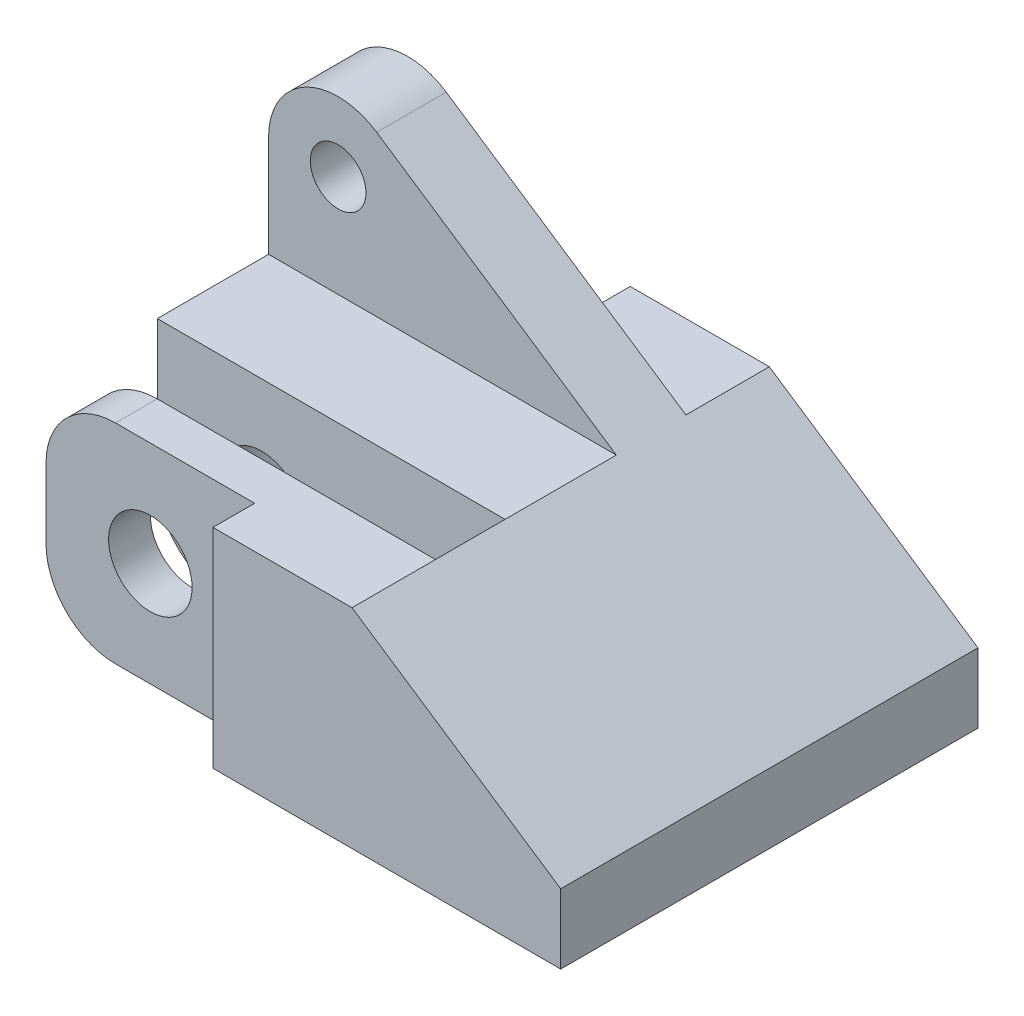
from build123d import *

# Parameters (mm, degrees)
BOSS_EXTRUDE1_DEPTH = 15
SKETCH2_W           = 38.199379203
SKETCH2_H           = 20.357752988
CUT_EXTRUDE1_DEPTH  = 30
SKETCH3_W           = 25
SKETCH3_H           = 5
CUT_EXTRUDE2_DEPTH  = 30
BOSS_EXTRUDE3_START = 6
SKETCH4_R           = 2
BOSS_EXTRUDE3_DEPTH = 5
SKETCH5_R           = 3
CUT_EXTRUDE3_DEPTH  = 27
FILLET1_R           = 5
FILLET2_R           = 5


with BuildPart() as part:
    # Sketch1 → Boss-Extrude1 (new, symmetric)
    with BuildSketch(Plane.XY):
        Polygon((0, 0), (0, 5), (-15, 15), (-40, 15), (-40, 0), align=None)
    extrude(amount=BOSS_EXTRUDE1_DEPTH, both=True)

    # Sketch2 → Cut-Extrude1 (cut)
    with BuildSketch(Plane(origin=(0, 15, 0), x_dir=(1, 0, 0), z_dir=(0, 1, 0))):
        with Locations((-44.099689602, 22.178876494)):
            Rectangle(SKETCH2_W, SKETCH2_H)
        with Locations((-44.099689602, -22.178876494)):
            Rectangle(SKETCH2_W, SKETCH2_H)
    extrude(amount=-CUT_EXTRUDE1_DEPTH, mode=Mode.SUBTRACT)

    # Sketch3 → Cut-Extrude2 (cut)
    with BuildSketch(Plane(origin=(0, 15, 0), x_dir=(1, 0, 0), z_dir=(0, 1, 0))):
        with Locations((-27.5, -6.5)):
            Rectangle(SKETCH3_W, SKETCH3_H)
    extrude(amount=-CUT_EXTRUDE2_DEPTH, mode=Mode.SUBTRACT)

    # Sketch4 → Boss-Extrude3 (add)
    with BuildSketch(Plane.XY.offset(-15).offset(BOSS_EXTRUDE3_START)):
        with BuildLine():
            Line((-15, 15), (-32.226499019, 26.484332679))
            ThreePointArc((-32.226499019, 26.484332679), (-37.359289628, 26.732454201), (-40, 22.324081208))
            Line((-40, 22.324081208), (-40, 15))
            Line((-40, 15), (-15, 15))
        make_face()
        with Locations((-35, 22.324081208)):
            Circle(SKETCH4_R, mode=Mode.SUBTRACT)
    extrude(amount=BOSS_EXTRUDE3_DEPTH)

    # Sketch5 → Cut-Extrude3 (cut)
    with BuildSketch(Plane.XY.offset(12)):
        with Locations((-32.5, 7.5)):
            Circle(SKETCH5_R)
    extrude(amount=-CUT_EXTRUDE3_DEPTH, mode=Mode.SUBTRACT)

    # Fillet1
    fillet1_edges = [part.edges().sort_by_distance(p)[0] for p in [
        (-40, 0, 10.5),
        (-40, 15, 10.5),
    ]]
    fillet(fillet1_edges, radius=FILLET1_R)

    # Fillet2
    fillet2_edges = [part.edges().sort_by_distance(p)[0] for p in [
        (-40, 0, -4),
    ]]
    fillet(fillet2_edges, radius=FILLET2_R)


solid = part.part
